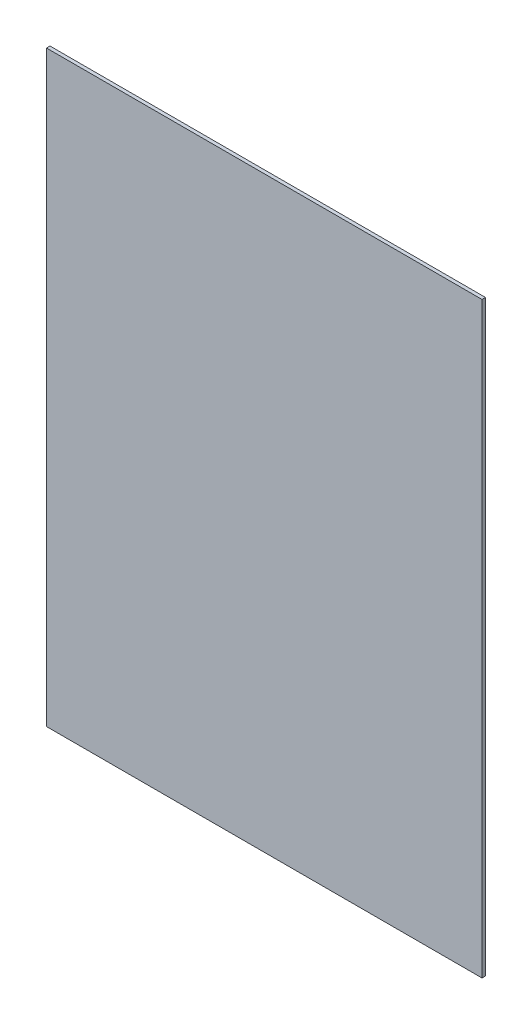
SolidWorks part; units mm, degrees
material "PMMA(有机玻璃)"
ref_plane "前视" through (0, 0, 0) normal (0, 0, 1) x (1, 0, 0)
ref_plane "上视" through (0, 0, 0) normal (0, 1, 0) x (1, 0, 0)
ref_plane "右视" through (0, 0, 0) normal (1, 0, 0) x (0, 0, -1)
sketch "草图1" plane through (0, 0, 0) normal (0, 0, 1) x (1, 0, 0)
  line L1 (-312, 421) -> (312, 421)
  line L2 (-312, 421) -> (-312, -421)
  line L3 (-312, -421) -> (312, -421)
  line L4 (312, 421) -> (312, -421)
  line L5 (-312, 421) -> (312, -421) construction
  line L6 (-312, -421) -> (312, 421) construction
  point P0 (0, 0)
  dimension "D1" = 842
  dimension "D2" = 624
extrude "凸台-拉伸1" add sketch "草图1" along normal blind 5
hole_wizard "M5 间隙孔1" positions "草图3" profile "草图2" hole size "M5" standard "GB"
sketch "草图3" plane through (0, 0, 5) normal (0, 0, 1) x (1, 0, 0)
  line L0 (-427.5, 273) -> (-427.5, -273) construction
  line L1 (-427.5, -273) -> (427.5, -273) construction
  line L2 (0, 273) -> (0, -273) construction
  line L3 (427.5, 273) -> (-427.5, 273) construction
  line L5 (-427.5, 0) -> (427.5, 0) construction
  line L6 (427.5, -273) -> (427.5, 273) construction
  point P0 (-375, -261)
  point P46 (415.5, 250)
  point P48 (-415.5, 250)
  point P58 (-125, -261)
  point P59 (125, -261)
  point P61 (-125, 261)
  point P62 (125, 261)
  point P64 (-375, 261)
  point P88 (375, -261)
  point P89 (375, 261)
  point P108 (415.5, 0)
  point P109 (-415.5, 0)
  point P110 (415.5, -250)
  point P111 (-415.5, -250)
  dimension "D1" = 12
  dimension "D2" = 12
  dimension "D5" = 3
  dimension "D3" = 12
  dimension "D6" = 4
  dimension "D4" = 2
sketch "草图2" plane through (-375, -261, 5) normal (1, 0, 0) x (0, -1, 0)
  line L0 (0, 0) -> (0, 5)
  line L1 (0, 5) -> (2.75, 5)
  line L2 (2.75, 5) -> (2.75, 0)
  line L5 (2.75, 0) -> (0, 0)
  line L11 (0, -6.35) -> (0, 107.95) construction
  dimension "通孔孔直径" = 5.5
  dimension "通孔孔深度" = 5
